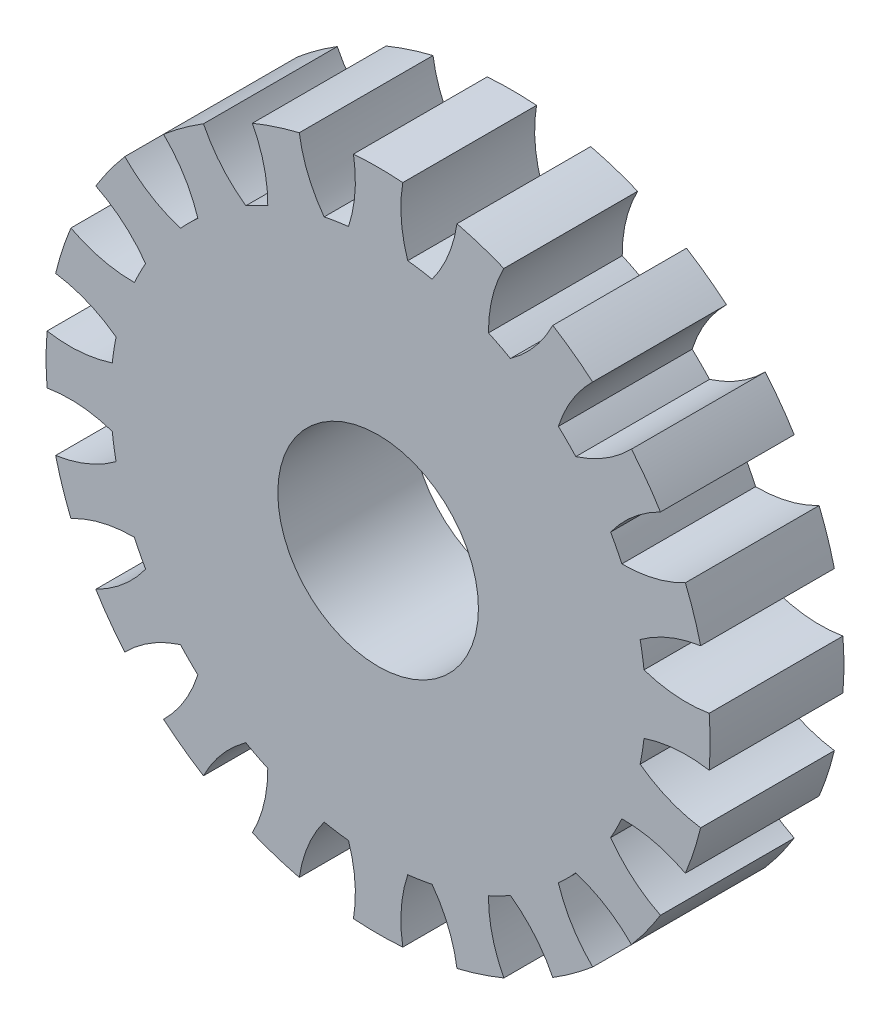
SolidWorks part; units mm, degrees
ref_plane "Front Plane" through (0, 0, 0) normal (0, 0, 1) x (1, 0, 0)
ref_plane "Top Plane" through (0, 0, 0) normal (0, 1, 0) x (1, 0, 0)
ref_plane "Right Plane" through (0, 0, 0) normal (1, 0, 0) x (0, 0, -1)
other "Configuration Table"
sketch "Sketch1" plane through (0, 0, 0) normal (0, 0, 1) x (1, 0, 0)
  circle A0 centre (0, 0) radius 40
  dimension "D1" = 80
extrude "Boss-Extrude1" add sketch "Sketch1" along normal mid plane 20
sketch "Sketch2" plane through (0, 0, 10) normal (0, 0, 1) x (1, 0, 0)
  circle A0 centre (0, 0) radius 15
  circle A1 centre (0, 0) radius 15 construction
extrude "Cut-Extrude1" cut sketch "Sketch2" against normal up to next contours A0
sketch "Sketch4" plane through (0, 0, 0) normal (0, 0, 1) x (1, 0, 0)
  line L0 (0, 50.836) -> (0, 0) construction
  arc A0 (3.9635, 50.836) -> (4.4294, 39.754) centre (23.5513, 46.1088) ccw
  arc A1 (-3.9635, 50.836) -> (-4.4294, 39.754) centre (-23.5513, 46.1088) cw
  circle A2 centre (0, 0) radius 40 construction
  arc A3 (4.4294, 39.754) -> (-4.4294, 39.754) centre (0, 0) ccw
  arc A4 (-3.9635, 50.836) -> (3.9635, 50.836) centre (0, 13.4287) cw
  dimension "D1" = 37.6167
extrude "Boss-Extrude2" add sketch "Sketch4" along normal mid plane 20
pattern_circular "CirPattern1" count 20 over 360 about axis through (0, 0, 0) along (0, 0, 1) of "Boss-Extrude2"
sketch "Sketch5" plane through (0, 0, -10) normal (0, 0, -1) x (-1, 0, 0)
  circle A0 centre (0, 0) radius 49.6406
extrude "Cut-Extrude4" cut sketch "Sketch5" against normal blind 53 flip side to cut
